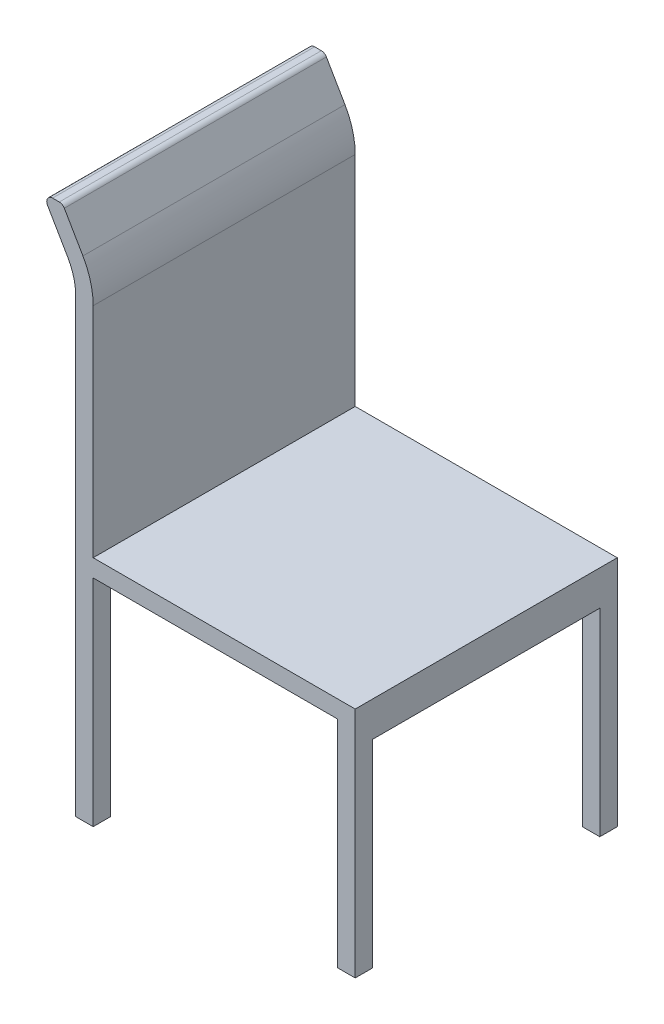
from build123d import *

# Parameters (mm, degrees)
BOSS_EXTRUDE1_DEPTH = 450
SKETCH2_W           = 390
SKETCH2_H           = 365.797461664
CUT_EXTRUDE1_DEPTH  = 500


with BuildPart() as part:
    # Sketch1 → Boss-Extrude1 (new body)
    with BuildSketch(Plane.XY):
        with BuildLine():
            Line((0, 0), (0, 774.761772336))
            ThreePointArc((0, 774.761772336), (-3.437744681, 800.756595814), (-13.514616953, 824.964147969))
            Line((-13.514616953, 824.964147969), (-48.352023173, 884.979762437))
            ThreePointArc((-48.352023173, 884.979762437), (-48.369579018, 894.989870959), (-39.703484868, 900))
            Line((-39.703484868, 900), (-28.140837346, 900))
            ThreePointArc((-28.140837346, 900), (-23.150966388, 898.66609415), (-19.492299041, 895.020237563))
            Line((-19.492299041, 895.020237563), (12.430997961, 840.024860659))
            ThreePointArc((12.430997961, 840.024860659), (25.530931915, 808.555042857), (30, 774.761772336))
            Line((30, 774.761772336), (30, 400))
            Line((30, 400), (480, 400))
            Line((480, 400), (480, 0))
            Line((480, 0), (450, 0))
            Line((450, 0), (450, 370))
            Line((450, 370), (30, 370))
            Line((30, 370), (30, 0))
            Line((30, 0), (0, 0))
        make_face()
    extrude(amount=BOSS_EXTRUDE1_DEPTH)

    # Sketch2 → Cut-Extrude1 (cut)
    with BuildSketch(Plane(origin=(480, 0, 0), x_dir=(0, 0, -1), z_dir=(1, 0, 0))):
        with Locations((-225, 157.101269168)):
            Rectangle(SKETCH2_W, SKETCH2_H)
    extrude(amount=-CUT_EXTRUDE1_DEPTH, mode=Mode.SUBTRACT)


solid = part.part
